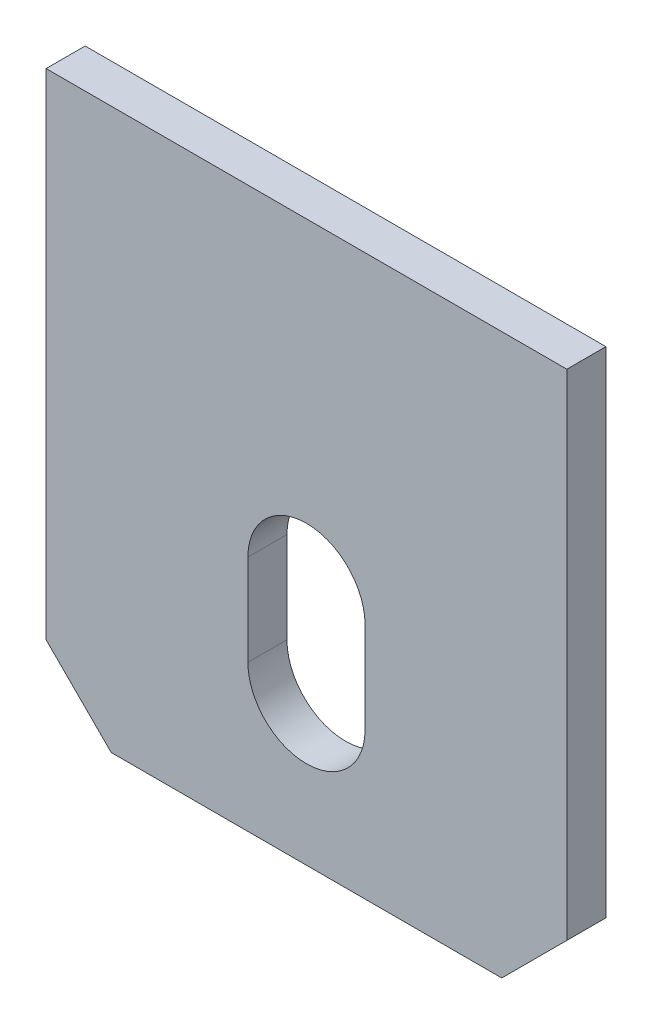
from build123d import *

# Parameters (mm, degrees)
BOSS_EXTRUDE1_DEPTH = 3


with BuildPart() as part:
    # Sketch1 → Boss-Extrude1 (new body)
    with BuildSketch(Plane.XY):
        Polygon((213.585362106, 213.495304552), (253.585362106, 213.495304552), (253.585362106, 175.495304552), (248.585362106, 170.495304552), (218.585362106, 170.495304552), (213.585362106, 175.495304552), align=None)
        with BuildLine():
            Line((229.085362106, 181.745304552), (229.085362106, 188.745304552))
            ThreePointArc((229.085362106, 188.745304552), (233.585362106, 193.245304552), (238.085362106, 188.745304552))
            Line((238.085362106, 188.745304552), (238.085362106, 181.745304552))
            ThreePointArc((238.085362106, 181.745304552), (233.585362106, 177.245304552), (229.085362106, 181.745304552))
        make_face(mode=Mode.SUBTRACT)
    extrude(amount=BOSS_EXTRUDE1_DEPTH)


solid = part.part
